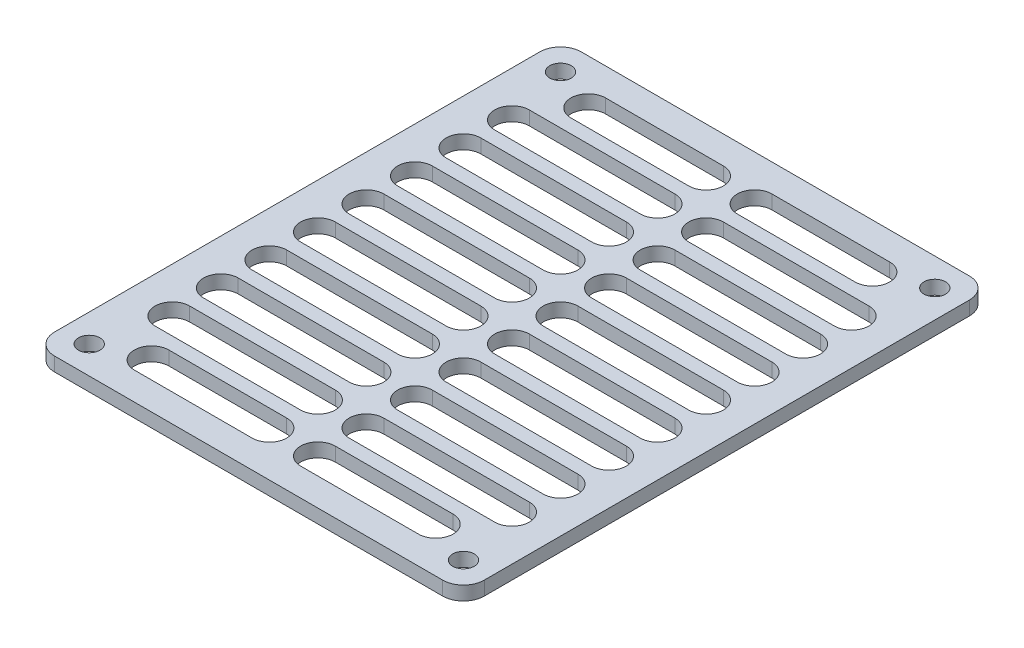
from build123d import *

# Parameters (mm, degrees)
SKETCH_1_W      = 62
SKETCH_1_H      = 76
SKETCH_1_R      = 1.55
EXTRUDE_1_DEPTH = 2
FILLET_1_R      = 3


with BuildPart() as part:
    # 草图1 → 凸台-拉伸1 (new body)
    with BuildSketch(Plane(origin=(0, 0, 0), x_dir=(1, 0, 0), z_dir=(0, 1, 0))):
        Rectangle(SKETCH_1_W, SKETCH_1_H)
        with Locations(Location((-27, -34, 0), (0, 0, 270))):
            Circle(SKETCH_1_R, mode=Mode.SUBTRACT)
        with BuildLine():
            ThreePointArc((-3.5, -29), (-1, -31.5), (-3.5, -34))
            Line((-3.5, -34), (-20.5, -34))
            ThreePointArc((-20.5, -34), (-23, -31.5), (-20.5, -29))
            Line((-20.5, -29), (-3.5, -29))
        make_face(mode=Mode.SUBTRACT)
        with BuildLine():
            ThreePointArc((-3.5, -22), (-1, -24.5), (-3.5, -27))
            Line((-3.5, -27), (-20.5, -27))
            Line((-20.5, -27), (-24.5, -27))
            ThreePointArc((-24.5, -27), (-27, -24.5), (-24.5, -22))
            Line((-24.5, -22), (-20.5, -22))
            Line((-20.5, -22), (-3.5, -22))
        make_face(mode=Mode.SUBTRACT)
        with BuildLine():
            ThreePointArc((-3.5, -15), (-1, -17.5), (-3.5, -20))
            Line((-3.5, -20), (-20.5, -20))
            Line((-20.5, -20), (-24.5, -20))
            ThreePointArc((-24.5, -20), (-27, -17.5), (-24.5, -15))
            Line((-24.5, -15), (-20.5, -15))
            Line((-20.5, -15), (-3.5, -15))
        make_face(mode=Mode.SUBTRACT)
        with BuildLine():
            ThreePointArc((-3.5, -8), (-1, -10.5), (-3.5, -13))
            Line((-3.5, -13), (-20.5, -13))
            Line((-20.5, -13), (-24.5, -13))
            ThreePointArc((-24.5, -13), (-27, -10.5), (-24.5, -8))
            Line((-24.5, -8), (-20.5, -8))
            Line((-20.5, -8), (-3.5, -8))
        make_face(mode=Mode.SUBTRACT)
        with BuildLine():
            ThreePointArc((-3.5, -1), (-1, -3.5), (-3.5, -6))
            Line((-3.5, -6), (-20.5, -6))
            Line((-20.5, -6), (-24.5, -6))
            ThreePointArc((-24.5, -6), (-27, -3.5), (-24.5, -1))
            Line((-24.5, -1), (-20.5, -1))
            Line((-20.5, -1), (-3.5, -1))
        make_face(mode=Mode.SUBTRACT)
        with BuildLine():
            Line((20.5, -34), (3.5, -34))
            ThreePointArc((3.5, -34), (1, -31.5), (3.5, -29))
            Line((3.5, -29), (20.5, -29))
            ThreePointArc((20.5, -29), (23, -31.5), (20.5, -34))
        make_face(mode=Mode.SUBTRACT)
        with BuildLine():
            Line((20.5, -27), (3.5, -27))
            ThreePointArc((3.5, -27), (1, -24.5), (3.5, -22))
            Line((3.5, -22), (20.5, -22))
            Line((20.5, -22), (24.5, -22))
            ThreePointArc((24.5, -22), (27, -24.5), (24.5, -27))
            Line((24.5, -27), (20.5, -27))
        make_face(mode=Mode.SUBTRACT)
        with Locations(Location((27, -34, 0), (0, 0, 270))):
            Circle(SKETCH_1_R, mode=Mode.SUBTRACT)
        with BuildLine():
            Line((20.5, -20), (3.5, -20))
            ThreePointArc((3.5, -20), (1, -17.5), (3.5, -15))
            Line((3.5, -15), (20.5, -15))
            Line((20.5, -15), (24.5, -15))
            ThreePointArc((24.5, -15), (27, -17.5), (24.5, -20))
            Line((24.5, -20), (20.5, -20))
        make_face(mode=Mode.SUBTRACT)
        with BuildLine():
            Line((20.5, -13), (3.5, -13))
            ThreePointArc((3.5, -13), (1, -10.5), (3.5, -8))
            Line((3.5, -8), (20.5, -8))
            Line((20.5, -8), (24.5, -8))
            ThreePointArc((24.5, -8), (27, -10.5), (24.5, -13))
            Line((24.5, -13), (20.5, -13))
        make_face(mode=Mode.SUBTRACT)
        with BuildLine():
            Line((20.5, -6), (3.5, -6))
            ThreePointArc((3.5, -6), (1, -3.5), (3.5, -1))
            Line((3.5, -1), (20.5, -1))
            Line((20.5, -1), (24.5, -1))
            ThreePointArc((24.5, -1), (27, -3.5), (24.5, -6))
            Line((24.5, -6), (20.5, -6))
        make_face(mode=Mode.SUBTRACT)
        with BuildLine():
            Line((-20.5, 6), (-3.5, 6))
            ThreePointArc((-3.5, 6), (-1, 3.5), (-3.5, 1))
            Line((-3.5, 1), (-20.5, 1))
            Line((-20.5, 1), (-24.5, 1))
            ThreePointArc((-24.5, 1), (-27, 3.5), (-24.5, 6))
            Line((-24.5, 6), (-20.5, 6))
        make_face(mode=Mode.SUBTRACT)
        with BuildLine():
            Line((-20.5, 13), (-3.5, 13))
            ThreePointArc((-3.5, 13), (-1, 10.5), (-3.5, 8))
            Line((-3.5, 8), (-20.5, 8))
            Line((-20.5, 8), (-24.5, 8))
            ThreePointArc((-24.5, 8), (-27, 10.5), (-24.5, 13))
            Line((-24.5, 13), (-20.5, 13))
        make_face(mode=Mode.SUBTRACT)
        with BuildLine():
            Line((-20.5, 20), (-3.5, 20))
            ThreePointArc((-3.5, 20), (-1, 17.5), (-3.5, 15))
            Line((-3.5, 15), (-20.5, 15))
            Line((-20.5, 15), (-24.5, 15))
            ThreePointArc((-24.5, 15), (-27, 17.5), (-24.5, 20))
            Line((-24.5, 20), (-20.5, 20))
        make_face(mode=Mode.SUBTRACT)
        with Locations(Location((-27, 34, 0), (0, 0, 270))):
            Circle(SKETCH_1_R, mode=Mode.SUBTRACT)
        with BuildLine():
            Line((-20.5, 27), (-3.5, 27))
            ThreePointArc((-3.5, 27), (-1, 24.5), (-3.5, 22))
            Line((-3.5, 22), (-20.5, 22))
            Line((-20.5, 22), (-24.5, 22))
            ThreePointArc((-24.5, 22), (-27, 24.5), (-24.5, 27))
            Line((-24.5, 27), (-20.5, 27))
        make_face(mode=Mode.SUBTRACT)
        with BuildLine():
            Line((-20.5, 34), (-3.5, 34))
            ThreePointArc((-3.5, 34), (-1, 31.5), (-3.5, 29))
            Line((-3.5, 29), (-20.5, 29))
            ThreePointArc((-20.5, 29), (-23, 31.5), (-20.5, 34))
        make_face(mode=Mode.SUBTRACT)
        with BuildLine():
            ThreePointArc((3.5, 1), (1, 3.5), (3.5, 6))
            Line((3.5, 6), (20.5, 6))
            Line((20.5, 6), (24.5, 6))
            ThreePointArc((24.5, 6), (27, 3.5), (24.5, 1))
            Line((24.5, 1), (20.5, 1))
            Line((20.5, 1), (3.5, 1))
        make_face(mode=Mode.SUBTRACT)
        with BuildLine():
            ThreePointArc((3.5, 8), (1, 10.5), (3.5, 13))
            Line((3.5, 13), (20.5, 13))
            Line((20.5, 13), (24.5, 13))
            ThreePointArc((24.5, 13), (27, 10.5), (24.5, 8))
            Line((24.5, 8), (20.5, 8))
            Line((20.5, 8), (3.5, 8))
        make_face(mode=Mode.SUBTRACT)
        with BuildLine():
            ThreePointArc((3.5, 15), (1, 17.5), (3.5, 20))
            Line((3.5, 20), (20.5, 20))
            Line((20.5, 20), (24.5, 20))
            ThreePointArc((24.5, 20), (27, 17.5), (24.5, 15))
            Line((24.5, 15), (20.5, 15))
            Line((20.5, 15), (3.5, 15))
        make_face(mode=Mode.SUBTRACT)
        with BuildLine():
            ThreePointArc((3.5, 22), (1, 24.5), (3.5, 27))
            Line((3.5, 27), (20.5, 27))
            Line((20.5, 27), (24.5, 27))
            ThreePointArc((24.5, 27), (27, 24.5), (24.5, 22))
            Line((24.5, 22), (20.5, 22))
            Line((20.5, 22), (3.5, 22))
        make_face(mode=Mode.SUBTRACT)
        with BuildLine():
            ThreePointArc((3.5, 29), (1, 31.5), (3.5, 34))
            Line((3.5, 34), (20.5, 34))
            ThreePointArc((20.5, 34), (23, 31.5), (20.5, 29))
            Line((20.5, 29), (3.5, 29))
        make_face(mode=Mode.SUBTRACT)
        with Locations(Location((27, 34, 0), (0, 0, 270))):
            Circle(SKETCH_1_R, mode=Mode.SUBTRACT)
    extrude(amount=EXTRUDE_1_DEPTH)

    # 圆角1
    fillet_1_edges = [part.edges().sort_by_distance(p)[0] for p in [
        (31, 1, -38),
        (31, 1, 38),
        (-31, 1, 38),
        (-31, 1, -38),
    ]]
    fillet(fillet_1_edges, radius=FILLET_1_R)


solid = part.part
